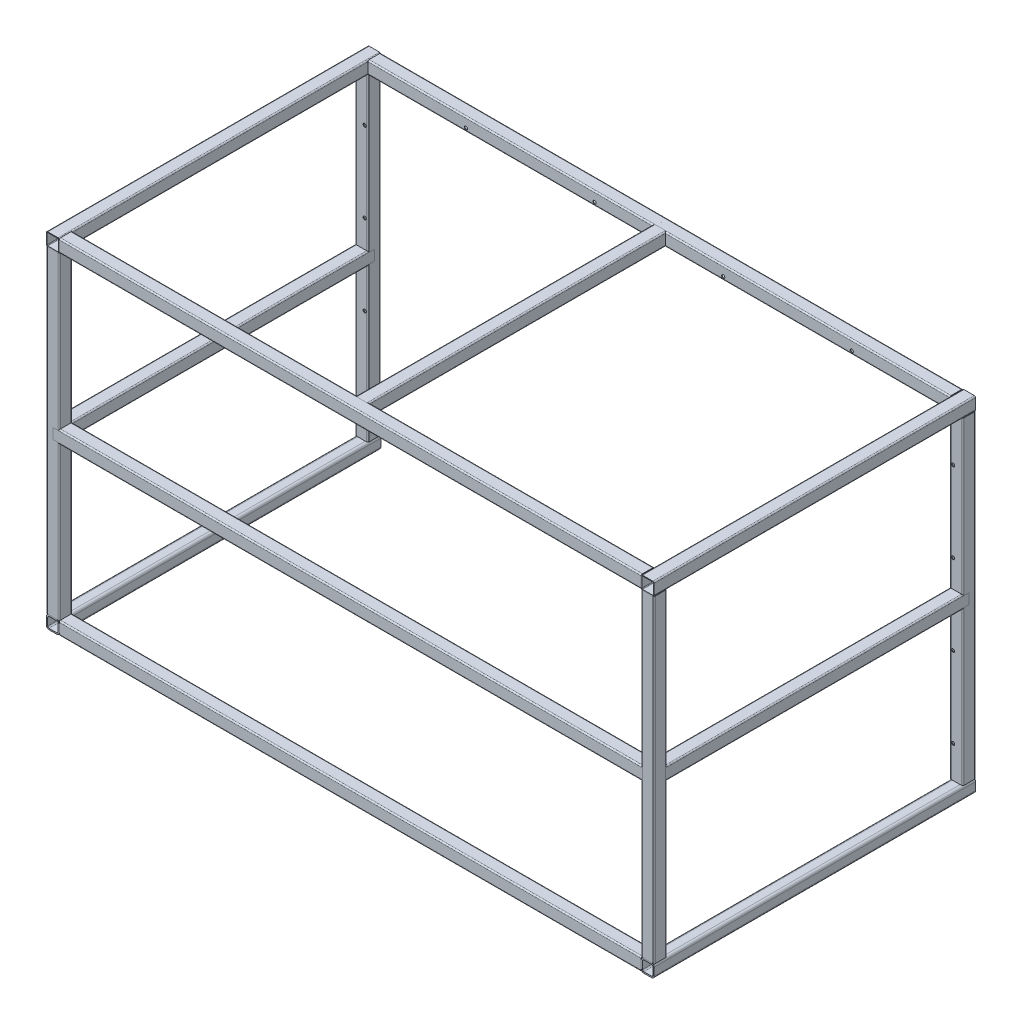
from build123d import *

# Parameters (mm, degrees)
SQUARE_TUBE_CONFIGURED_40_X_40_X_4_1_DEPTH      = 1870
SQUARE_TUBE_CONFIGURED_40_X_40_X_4_1_DEPTH_BACK = 1
SQUARE_TUBE_CONFIGURED_40_X_40_X_4_1_2_DEPTH    = 1051
SQUARE_TUBE_CONFIGURED_40_X_40_X_4_1_3_DEPTH    = 1871
SQUARE_TUBE_CONFIGURED_40_X_40_X_4_1_4_DEPTH    = 1051
SQUARE_TUBE_CONFIGURED_40_X_40_X_4_5_DEPTH      = 1050
SQUARE_TUBE_CONFIGURED_40_X_40_X_4_5_2_DEPTH    = 1871
SQUARE_TUBE_CONFIGURED_40_X_40_X_4_5_3_DEPTH    = 1031
SQUARE_TUBE_CONFIGURED_40_X_40_X_4_8_DEPTH      = 960
SQUARE_TUBE_CONFIGURED_40_X_40_X_4_8_2_DEPTH    = 960
BODY_START                                      = 134.13708499
BODY_4_RUN_ON_DEPTH                             = 153.13708499
BODY_7_RUN_ON_DEPTH                             = 153.13708499
BODY_2_RUN_ON_DEPTH                             = 153.13708499
BODY_START_2                                    = 113.13708499
BODY_8_RUN_ON_DEPTH                             = 133.13708499
BODY_START_3                                    = 846.86291501
BODY_8_RUN_ON_2_DEPTH                           = 133.13708499
BODY_9_RUN_ON_DEPTH                             = 133.13708499
BODY_9_RUN_ON_2_DEPTH                           = 133.13708499
SQUARE_TUBE_CONFIGURED_40_X_40_X_4_9_DEPTH      = 960
SQUARE_TUBE_CONFIGURED_40_X_40_X_4_10_DEPTH     = 1850
SQUARE_TUBE_CONFIGURED_40_X_40_X_4_11_DEPTH     = 960
SQUARE_TUBE_CONFIGURED_40_X_40_X_4_12_DEPTH     = 960
SQUARE_TUBE_CONFIGURED_40_X_40_X_4_13_DEPTH     = 670
SQUARE_TUBE_CONFIGURED_40_X_40_X_4_14_DEPTH     = 670
BODY_14_RUN_ON_DEPTH                            = 20
BODY_15_RUN_ON_DEPTH                            = 20
BODY_START_4                                    = 670
BODY_14_RUN_ON_2_DEPTH                          = 310
BODY_15_RUN_ON_2_DEPTH                          = 310
SKETCH_4_W                                      = 5
SKETCH_4_H                                      = 40
PATTERN_LINEAR_1_COUNT                          = 4
PATTERN_LINEAR_1_PITCH                          = 250
PATTERN_LINEAR_2_COUNT                          = 2
PATTERN_LINEAR_2_PITCH                          = 1830
PATTERN_LINEAR_2_COPY_1_SKETCH_W                = 5
PATTERN_LINEAR_2_COPY_1_SKETCH_H                = 40
PATTERN_LINEAR_2_COPY_2_SKETCH_W                = 5
PATTERN_LINEAR_2_COPY_2_SKETCH_H                = 40
PATTERN_LINEAR_2_COPY_3_SKETCH_W                = 5
PATTERN_LINEAR_2_COPY_3_SKETCH_H                = 40
SKETCH_6_W                                      = 5
SKETCH_6_H                                      = 40
PATTERN_LINEAR_3_COUNT                          = 4
PATTERN_LINEAR_3_PITCH                          = 400


with BuildPart() as part:
    # Sketch1 → Square tube - configured 40 X 40 X 4(1) (new, two sides: drawn at the far end of the back side and taken through both)
    with BuildSketch(Plane(origin=(-925, 515, 0), x_dir=(0, 1, 0), z_dir=(1, 0, 0)).offset(-SQUARE_TUBE_CONFIGURED_40_X_40_X_4_1_DEPTH_BACK)):
        with BuildLine():
            Line((-16, -20), (16, -20))
            ThreePointArc((16, -20), (18.828427125, -18.828427125), (20, -16))
            Line((20, -16), (20, 16))
            ThreePointArc((20, 16), (18.828427125, 18.828427125), (16, 20))
            Line((16, 20), (-16, 20))
            ThreePointArc((-16, 20), (-18.828427125, 18.828427125), (-20, 16))
            Line((-20, 16), (-20, -16))
            ThreePointArc((-20, -16), (-18.828427125, -18.828427125), (-16, -20))
        make_face()
        with BuildLine():
            Line((-16, -18), (16, -18))
            ThreePointArc((16, -18), (17.414213562, -17.414213562), (18, -16))
            Line((18, -16), (18, 16))
            ThreePointArc((18, 16), (17.414213562, 17.414213562), (16, 18))
            Line((16, 18), (-16, 18))
            ThreePointArc((-16, 18), (-17.414213562, 17.414213562), (-18, 16))
            Line((-18, 16), (-18, -16))
            ThreePointArc((-18, -16), (-17.414213562, -17.414213562), (-16, -18))
        make_face(mode=Mode.SUBTRACT)
    extrude(amount=SQUARE_TUBE_CONFIGURED_40_X_40_X_4_1_DEPTH + SQUARE_TUBE_CONFIGURED_40_X_40_X_4_1_DEPTH_BACK)

    # Square tube - configured 40 X 40 X 4(1) e
    split(bisect_by=Plane(origin=(-905, 515, 0), x_dir=(0, 1, 0), z_dir=(1, 0, 0)), keep=Keep.TOP)

    # Weld Trim 17 7
    split(bisect_by=Plane(origin=(943, -20, 0), x_dir=(0, -1, 0), z_dir=(-1, 0, 0)), keep=Keep.TOP)

    # Weld Trim 17 12
    split(bisect_by=Plane(origin=(907, -20, 0), x_dir=(0, -1, 0), z_dir=(-1, 0, 0)), keep=Keep.TOP)

    # Weld Trim 17 13
    split(bisect_by=Plane(origin=(905, -20, 0), x_dir=(0, -1, 0), z_dir=(-1, 0, 0)), keep=Keep.TOP)


with BuildPart() as body_2:
    # Sketch1 on segment 2 (carried to segment 2) → Square tube - configured 40 X 40 X 4_1 2 (new body)
    with BuildSketch(Plane(origin=(925, 516, 0), x_dir=(1, 0, 0), z_dir=(0, -1, 0))):
        with BuildLine():
            Line((-16, -20), (16, -20))
            ThreePointArc((16, -20), (18.828427125, -18.828427125), (20, -16))
            Line((20, -16), (20, 16))
            ThreePointArc((20, 16), (18.828427125, 18.828427125), (16, 20))
            Line((16, 20), (-16, 20))
            ThreePointArc((-16, 20), (-18.828427125, 18.828427125), (-20, 16))
            Line((-20, 16), (-20, -16))
            ThreePointArc((-20, -16), (-18.828427125, -18.828427125), (-16, -20))
        make_face()
        with BuildLine():
            Line((-16, -18), (16, -18))
            ThreePointArc((16, -18), (17.414213562, -17.414213562), (18, -16))
            Line((18, -16), (18, 16))
            ThreePointArc((18, 16), (17.414213562, 17.414213562), (16, 18))
            Line((16, 18), (-16, 18))
            ThreePointArc((-16, 18), (-17.414213562, 17.414213562), (-18, 16))
            Line((-18, 16), (-18, -16))
            ThreePointArc((-18, -16), (-17.414213562, -17.414213562), (-16, -18))
        make_face(mode=Mode.SUBTRACT)
    extrude(amount=SQUARE_TUBE_CONFIGURED_40_X_40_X_4_1_2_DEPTH)

    # Square tube - configured 40 X 40 X 4 2
    split(bisect_by=Plane(origin=(925, 495, 0), x_dir=(1, 0, 0), z_dir=(0, -1, 0)), keep=Keep.TOP)

    # body 2 cut square before the run-on
    split(bisect_by=Plane(origin=(925, 381.86291501, 0), x_dir=(1, 0, 0), z_dir=(0, -1, 0)), keep=Keep.TOP)

    # Sketch1 on segment 2 (carried to segment 2) → body 2 run on (add)
    with BuildSketch(Plane(origin=(925, 516, 0), x_dir=(1, 0, 0), z_dir=(0, -1, 0)).offset(BODY_START)):
        with BuildLine():
            Line((-16, -20), (16, -20))
            ThreePointArc((16, -20), (18.828427125, -18.828427125), (20, -16))
            Line((20, -16), (20, 16))
            ThreePointArc((20, 16), (18.828427125, 18.828427125), (16, 20))
            Line((16, 20), (-16, 20))
            ThreePointArc((-16, 20), (-18.828427125, 18.828427125), (-20, 16))
            Line((-20, 16), (-20, -16))
            ThreePointArc((-20, -16), (-18.828427125, -18.828427125), (-16, -20))
        make_face()
        with BuildLine():
            Line((-16, -18), (16, -18))
            ThreePointArc((16, -18), (17.414213562, -17.414213562), (18, -16))
            Line((18, -16), (18, 16))
            ThreePointArc((18, 16), (17.414213562, 17.414213562), (16, 18))
            Line((16, 18), (-16, 18))
            ThreePointArc((-16, 18), (-17.414213562, 17.414213562), (-18, 16))
            Line((-18, 16), (-18, -16))
            ThreePointArc((-18, -16), (-17.414213562, -17.414213562), (-16, -18))
        make_face(mode=Mode.SUBTRACT)
    extrude(amount=-BODY_2_RUN_ON_DEPTH)

    # Weld Trim 25 5
    split(bisect_by=Plane(origin=(925, 495, -490), x_dir=(1, 0, 0), z_dir=(0, -1, 0)), keep=Keep.TOP)

    # Weld Trim 32
    split(bisect_by=Plane(origin=(925, -495, -335), x_dir=(-1, 0, 0), z_dir=(0, 1, 0)), keep=Keep.TOP)


with BuildPart() as body_3:
    # Sketch1 on segment 3 (carried to segment 3) → Square tube - configured 40 X 40 X 4_1 3 (new body)
    with BuildSketch(Plane(origin=(926, -515, 0), x_dir=(0, -1, 0), z_dir=(-1, 0, 0))):
        with BuildLine():
            Line((-16, -20), (16, -20))
            ThreePointArc((16, -20), (18.828427125, -18.828427125), (20, -16))
            Line((20, -16), (20, 16))
            ThreePointArc((20, 16), (18.828427125, 18.828427125), (16, 20))
            Line((16, 20), (-16, 20))
            ThreePointArc((-16, 20), (-18.828427125, 18.828427125), (-20, 16))
            Line((-20, 16), (-20, -16))
            ThreePointArc((-20, -16), (-18.828427125, -18.828427125), (-16, -20))
        make_face()
        with BuildLine():
            Line((-16, -18), (16, -18))
            ThreePointArc((16, -18), (17.414213562, -17.414213562), (18, -16))
            Line((18, -16), (18, 16))
            ThreePointArc((18, 16), (17.414213562, 17.414213562), (16, 18))
            Line((16, 18), (-16, 18))
            ThreePointArc((-16, 18), (-17.414213562, 17.414213562), (-18, 16))
            Line((-18, 16), (-18, -16))
            ThreePointArc((-18, -16), (-17.414213562, -17.414213562), (-16, -18))
        make_face(mode=Mode.SUBTRACT)
    extrude(amount=SQUARE_TUBE_CONFIGURED_40_X_40_X_4_1_3_DEPTH)

    # Square tube - configured 40 X 40 X 4 3
    split(bisect_by=Plane(origin=(905, -515, 0), x_dir=(0, -1, 0), z_dir=(-1, 0, 0)), keep=Keep.TOP)

    # Weld Trim 1 7
    split(bisect_by=Plane(origin=(-943, 20, 0), x_dir=(0, 1, 0), z_dir=(1, 0, 0)), keep=Keep.TOP)

    # Weld Trim 1 12
    split(bisect_by=Plane(origin=(-907, 20, 0), x_dir=(0, 1, 0), z_dir=(1, 0, 0)), keep=Keep.TOP)

    # Weld Trim 1 13
    split(bisect_by=Plane(origin=(-905, 20, 0), x_dir=(0, 1, 0), z_dir=(1, 0, 0)), keep=Keep.TOP)


with BuildPart() as body_4:
    # Sketch1 on segment 4 (carried to segment 4) → Square tube - configured 40 X 40 X 4_1 4 (new body)
    with BuildSketch(Plane(origin=(-925, -516, 0), x_dir=(-1, 0, 0), z_dir=(0, 1, 0))):
        with BuildLine():
            Line((-16, -20), (16, -20))
            ThreePointArc((16, -20), (18.828427125, -18.828427125), (20, -16))
            Line((20, -16), (20, 16))
            ThreePointArc((20, 16), (18.828427125, 18.828427125), (16, 20))
            Line((16, 20), (-16, 20))
            ThreePointArc((-16, 20), (-18.828427125, 18.828427125), (-20, 16))
            Line((-20, 16), (-20, -16))
            ThreePointArc((-20, -16), (-18.828427125, -18.828427125), (-16, -20))
        make_face()
        with BuildLine():
            Line((-16, -18), (16, -18))
            ThreePointArc((16, -18), (17.414213562, -17.414213562), (18, -16))
            Line((18, -16), (18, 16))
            ThreePointArc((18, 16), (17.414213562, 17.414213562), (16, 18))
            Line((16, 18), (-16, 18))
            ThreePointArc((-16, 18), (-17.414213562, 17.414213562), (-18, 16))
            Line((-18, 16), (-18, -16))
            ThreePointArc((-18, -16), (-17.414213562, -17.414213562), (-16, -18))
        make_face(mode=Mode.SUBTRACT)
    extrude(amount=SQUARE_TUBE_CONFIGURED_40_X_40_X_4_1_4_DEPTH)

    # Square tube - configured 40 X 40 X 4 4
    split(bisect_by=Plane(origin=(-925, -495, 0), x_dir=(-1, 0, 0), z_dir=(0, 1, 0)), keep=Keep.TOP)

    # body 4 cut square before the run-on
    split(bisect_by=Plane(origin=(-925, -381.86291501, 0), x_dir=(-1, 0, 0), z_dir=(0, 1, 0)), keep=Keep.TOP)

    # Sketch1 on segment 4 (carried to segment 4) → body 4 run on (add)
    with BuildSketch(Plane(origin=(-925, -516, 0), x_dir=(-1, 0, 0), z_dir=(0, 1, 0)).offset(BODY_START)):
        with BuildLine():
            Line((-16, -20), (16, -20))
            ThreePointArc((16, -20), (18.828427125, -18.828427125), (20, -16))
            Line((20, -16), (20, 16))
            ThreePointArc((20, 16), (18.828427125, 18.828427125), (16, 20))
            Line((16, 20), (-16, 20))
            ThreePointArc((-16, 20), (-18.828427125, 18.828427125), (-20, 16))
            Line((-20, 16), (-20, -16))
            ThreePointArc((-20, -16), (-18.828427125, -18.828427125), (-16, -20))
        make_face()
        with BuildLine():
            Line((-16, -18), (16, -18))
            ThreePointArc((16, -18), (17.414213562, -17.414213562), (18, -16))
            Line((18, -16), (18, 16))
            ThreePointArc((18, 16), (17.414213562, 17.414213562), (16, 18))
            Line((16, 18), (-16, 18))
            ThreePointArc((-16, 18), (-17.414213562, 17.414213562), (-18, 16))
            Line((-18, 16), (-18, -16))
            ThreePointArc((-18, -16), (-17.414213562, -17.414213562), (-16, -18))
        make_face(mode=Mode.SUBTRACT)
    extrude(amount=-BODY_4_RUN_ON_DEPTH)

    # Weld Trim 18 5
    split(bisect_by=Plane(origin=(-925, 495, -480), x_dir=(1, 0, 0), z_dir=(0, -1, 0)), keep=Keep.TOP)

    # Weld Trim 31
    split(bisect_by=Plane(origin=(-925, -495, -335), x_dir=(-1, 0, 0), z_dir=(0, 1, 0)), keep=Keep.TOP)


with BuildPart() as body_5:
    # Sketch11 → Square tube - configured 40 X 40 X 4 5 (new body)
    with BuildSketch(Plane(origin=(925, -515, -960), x_dir=(-1, 0, 0), z_dir=(0, 1, 0))):
        with BuildLine():
            Line((-16, -20), (16, -20))
            ThreePointArc((16, -20), (18.828427125, -18.828427125), (20, -16))
            Line((20, -16), (20, 16))
            ThreePointArc((20, 16), (18.828427125, 18.828427125), (16, 20))
            Line((16, 20), (-16, 20))
            ThreePointArc((-16, 20), (-18.828427125, 18.828427125), (-20, 16))
            Line((-20, 16), (-20, -16))
            ThreePointArc((-20, -16), (-18.828427125, -18.828427125), (-16, -20))
        make_face()
        with BuildLine():
            Line((-16, -18), (16, -18))
            ThreePointArc((16, -18), (17.414213562, -17.414213562), (18, -16))
            Line((18, -16), (18, 16))
            ThreePointArc((18, 16), (17.414213562, 17.414213562), (16, 18))
            Line((16, 18), (-16, 18))
            ThreePointArc((-16, 18), (-17.414213562, 17.414213562), (-18, 16))
            Line((-18, 16), (-18, -16))
            ThreePointArc((-18, -16), (-17.414213562, -17.414213562), (-16, -18))
        make_face(mode=Mode.SUBTRACT)
    extrude(amount=SQUARE_TUBE_CONFIGURED_40_X_40_X_4_5_DEPTH)

    # Weld Trim 23 5
    split(bisect_by=Plane(origin=(925, 495, -480), x_dir=(1, 0, 0), z_dir=(0, -1, 0)), keep=Keep.TOP)

    # Weld Trim 34
    split(bisect_by=Plane(origin=(925, -495, -325), x_dir=(-1, 0, 0), z_dir=(0, 1, 0)), keep=Keep.TOP)

    # 草图4 → Ø10.0 (10) 直径孔1 (revolve, cut)
    with BuildSketch(Plane(origin=(915, -395, -940), x_dir=(0, -1, 0), z_dir=(1, 0, 0))):
        with Locations((2.5, 20)):
            Rectangle(SKETCH_4_W, SKETCH_4_H)
    hole_wizard_10_0_10_1 = revolve(axis=Axis((915, -395, -933.65), (0, 0, -1)), mode=Mode.SUBTRACT)

    # 阵列(线性)1: Ø10.0 (10) 直径孔1 ×4
    with Locations(*[(0, i * PATTERN_LINEAR_1_PITCH, 0) for i in range(1, PATTERN_LINEAR_1_COUNT)]):
        add(hole_wizard_10_0_10_1, mode=Mode.SUBTRACT)


with BuildPart() as body_6:
    # Sketch11 on segment 2 (carried to segment 2) → Square tube - configured 40 X 40 X 4 5 2 (new body)
    with BuildSketch(Plane(origin=(926, 515, -960), x_dir=(0, -1, 0), z_dir=(-1, 0, 0))):
        with BuildLine():
            Line((-16, -20), (16, -20))
            ThreePointArc((16, -20), (18.828427125, -18.828427125), (20, -16))
            Line((20, -16), (20, 16))
            ThreePointArc((20, 16), (18.828427125, 18.828427125), (16, 20))
            Line((16, 20), (-16, 20))
            ThreePointArc((-16, 20), (-18.828427125, 18.828427125), (-20, 16))
            Line((-20, 16), (-20, -16))
            ThreePointArc((-20, -16), (-18.828427125, -18.828427125), (-16, -20))
        make_face()
        with BuildLine():
            Line((-16, -18), (16, -18))
            ThreePointArc((16, -18), (17.414213562, -17.414213562), (18, -16))
            Line((18, -16), (18, 16))
            ThreePointArc((18, 16), (17.414213562, 17.414213562), (16, 18))
            Line((16, 18), (-16, 18))
            ThreePointArc((-16, 18), (-17.414213562, 17.414213562), (-18, 16))
            Line((-18, 16), (-18, -16))
            ThreePointArc((-18, -16), (-17.414213562, -17.414213562), (-16, -18))
        make_face(mode=Mode.SUBTRACT)
    extrude(amount=SQUARE_TUBE_CONFIGURED_40_X_40_X_4_5_2_DEPTH)

    # Square tube - configured 40 X 40 X 4 6
    split(bisect_by=Plane(origin=(905, 515, -960), x_dir=(0, -1, 0), z_dir=(-1, 0, 0)), keep=Keep.TOP)

    # Weld Trim 5 7
    split(bisect_by=Plane(origin=(-905, -10, -960), x_dir=(0, 1, 0), z_dir=(1, 0, 0)), keep=Keep.TOP)

    # 草图6 → Ø10.0 (10) 直径孔2 (revolve, cut)
    with BuildSketch(Plane(origin=(600, 505, -940), x_dir=(0, -1, 0), z_dir=(1, 0, 0))):
        with Locations((2.5, 20)):
            Rectangle(SKETCH_6_W, SKETCH_6_H)
    hole_wizard_10_0_10_2 = revolve(axis=Axis((600, 505, -933.65), (0, 0, -1)), mode=Mode.SUBTRACT)

    # 阵列(线性)3: Ø10.0 (10) 直径孔2 ×4
    with Locations(*[(-i * PATTERN_LINEAR_3_PITCH, 0, 0) for i in range(1, PATTERN_LINEAR_3_COUNT)]):
        add(hole_wizard_10_0_10_2, mode=Mode.SUBTRACT)


with BuildPart() as body_7:
    # Sketch11 on segment 3 (carried to segment 3) → Square tube - configured 40 X 40 X 4 5 3 (new body)
    with BuildSketch(Plane(origin=(-925, 516, -960), x_dir=(1, 0, 0), z_dir=(0, -1, 0))):
        with BuildLine():
            Line((-16, -20), (16, -20))
            ThreePointArc((16, -20), (18.828427125, -18.828427125), (20, -16))
            Line((20, -16), (20, 16))
            ThreePointArc((20, 16), (18.828427125, 18.828427125), (16, 20))
            Line((16, 20), (-16, 20))
            ThreePointArc((-16, 20), (-18.828427125, 18.828427125), (-20, 16))
            Line((-20, 16), (-20, -16))
            ThreePointArc((-20, -16), (-18.828427125, -18.828427125), (-16, -20))
        make_face()
        with BuildLine():
            Line((-16, -18), (16, -18))
            ThreePointArc((16, -18), (17.414213562, -17.414213562), (18, -16))
            Line((18, -16), (18, 16))
            ThreePointArc((18, 16), (17.414213562, 17.414213562), (16, 18))
            Line((16, 18), (-16, 18))
            ThreePointArc((-16, 18), (-17.414213562, 17.414213562), (-18, 16))
            Line((-18, 16), (-18, -16))
            ThreePointArc((-18, -16), (-17.414213562, -17.414213562), (-16, -18))
        make_face(mode=Mode.SUBTRACT)
    extrude(amount=SQUARE_TUBE_CONFIGURED_40_X_40_X_4_5_3_DEPTH)

    # Square tube - configured 40 X 40 X 4 7
    split(bisect_by=Plane(origin=(-925, 495, -960), x_dir=(1, 0, 0), z_dir=(0, -1, 0)), keep=Keep.TOP)

    # body 7 cut square before the run-on
    split(bisect_by=Plane(origin=(-925, 381.86291501, -960), x_dir=(1, 0, 0), z_dir=(0, -1, 0)), keep=Keep.TOP)

    # Sketch11 on segment 3 (carried to segment 3) → body 7 run on (add)
    with BuildSketch(Plane(origin=(-925, 516, -960), x_dir=(1, 0, 0), z_dir=(0, -1, 0)).offset(BODY_START)):
        with BuildLine():
            Line((-16, -20), (16, -20))
            ThreePointArc((16, -20), (18.828427125, -18.828427125), (20, -16))
            Line((20, -16), (20, 16))
            ThreePointArc((20, 16), (18.828427125, 18.828427125), (16, 20))
            Line((16, 20), (-16, 20))
            ThreePointArc((-16, 20), (-18.828427125, 18.828427125), (-20, 16))
            Line((-20, 16), (-20, -16))
            ThreePointArc((-20, -16), (-18.828427125, -18.828427125), (-16, -20))
        make_face()
        with BuildLine():
            Line((-16, -18), (16, -18))
            ThreePointArc((16, -18), (17.414213562, -17.414213562), (18, -16))
            Line((18, -16), (18, 16))
            ThreePointArc((18, 16), (17.414213562, 17.414213562), (16, 18))
            Line((16, 18), (-16, 18))
            ThreePointArc((-16, 18), (-17.414213562, 17.414213562), (-18, 16))
            Line((-18, 16), (-18, -16))
            ThreePointArc((-18, -16), (-17.414213562, -17.414213562), (-16, -18))
        make_face(mode=Mode.SUBTRACT)
    extrude(amount=-BODY_7_RUN_ON_DEPTH)

    # Weld Trim 22 3
    split(bisect_by=Plane(origin=(-925, 533, -470), x_dir=(1, 0, 0), z_dir=(0, -1, 0)), keep=Keep.TOP)

    # Weld Trim 22 8
    split(bisect_by=Plane(origin=(-925, 497, -470), x_dir=(1, 0, 0), z_dir=(0, -1, 0)), keep=Keep.TOP)

    # Weld Trim 22 13
    split(bisect_by=Plane(origin=(-925, 495, -470), x_dir=(1, 0, 0), z_dir=(0, -1, 0)), keep=Keep.TOP)

    # Weld Trim 33
    split(bisect_by=Plane(origin=(-925, -495, -325), x_dir=(-1, 0, 0), z_dir=(0, 1, 0)), keep=Keep.TOP)

    # 阵列(线性)2: Ø10.0 (10) 直径孔1 ×2
    with Locations(*[(-i * PATTERN_LINEAR_2_PITCH, 0, 0) for i in range(1, PATTERN_LINEAR_2_COUNT)]):
        add(hole_wizard_10_0_10_1, mode=Mode.SUBTRACT)

    # 阵列(线性)2 copy 1 sketch → 阵列(线性)2 copy 1 (revolve, cut)
    with BuildSketch(Plane(origin=(-915, -145, -940), x_dir=(0, -1, 0), z_dir=(1, 0, 0))):
        with Locations((2.5, 20)):
            Rectangle(PATTERN_LINEAR_2_COPY_1_SKETCH_W, PATTERN_LINEAR_2_COPY_1_SKETCH_H)
    revolve(axis=Axis((-915, -145, -933.65), (0, 0, -1)), mode=Mode.SUBTRACT)

    # 阵列(线性)2 copy 2 sketch → 阵列(线性)2 copy 2 (revolve, cut)
    with BuildSketch(Plane(origin=(-915, 105, -940), x_dir=(0, -1, 0), z_dir=(1, 0, 0))):
        with Locations((2.5, 20)):
            Rectangle(PATTERN_LINEAR_2_COPY_2_SKETCH_W, PATTERN_LINEAR_2_COPY_2_SKETCH_H)
    revolve(axis=Axis((-915, 105, -933.65), (0, 0, -1)), mode=Mode.SUBTRACT)

    # 阵列(线性)2 copy 3 sketch → 阵列(线性)2 copy 3 (revolve, cut)
    with BuildSketch(Plane(origin=(-915, 355, -940), x_dir=(0, -1, 0), z_dir=(1, 0, 0))):
        with Locations((2.5, 20)):
            Rectangle(PATTERN_LINEAR_2_COPY_3_SKETCH_W, PATTERN_LINEAR_2_COPY_3_SKETCH_H)
    revolve(axis=Axis((-915, 355, -933.65), (0, 0, -1)), mode=Mode.SUBTRACT)


with BuildPart() as body_8:
    # Sketch12 → Square tube - configured 40 X 40 X 4 8 (new body)
    with BuildSketch(Plane(origin=(-925, 515, 0), x_dir=(1, 0, 0), z_dir=(0, 0, -1))):
        with BuildLine():
            Line((-16, -20), (16, -20))
            ThreePointArc((16, -20), (18.828427125, -18.828427125), (20, -16))
            Line((20, -16), (20, 16))
            ThreePointArc((20, 16), (18.828427125, 18.828427125), (16, 20))
            Line((16, 20), (-16, 20))
            ThreePointArc((-16, 20), (-18.828427125, 18.828427125), (-20, 16))
            Line((-20, 16), (-20, -16))
            ThreePointArc((-20, -16), (-18.828427125, -18.828427125), (-16, -20))
        make_face()
        with BuildLine():
            Line((-16, -18), (16, -18))
            ThreePointArc((16, -18), (17.414213562, -17.414213562), (18, -16))
            Line((18, -16), (18, 16))
            ThreePointArc((18, 16), (17.414213562, 17.414213562), (16, 18))
            Line((16, 18), (-16, 18))
            ThreePointArc((-16, 18), (-17.414213562, 17.414213562), (-18, 16))
            Line((-18, 16), (-18, -16))
            ThreePointArc((-18, -16), (-17.414213562, -17.414213562), (-16, -18))
        make_face(mode=Mode.SUBTRACT)
    extrude(amount=SQUARE_TUBE_CONFIGURED_40_X_40_X_4_8_DEPTH)

    # body 8 cut square before the run-on
    split(bisect_by=Plane(origin=(-925, 515, -113.13708499), x_dir=(0, 1, 0), z_dir=(0, 0, -1)), keep=Keep.TOP)

    # Sketch12 → body 8 run on (add)
    with BuildSketch(Plane(origin=(-925, 515, 0), x_dir=(1, 0, 0), z_dir=(0, 0, -1)).offset(BODY_START_2)):
        with BuildLine():
            Line((-16, -20), (16, -20))
            ThreePointArc((16, -20), (18.828427125, -18.828427125), (20, -16))
            Line((20, -16), (20, 16))
            ThreePointArc((20, 16), (18.828427125, 18.828427125), (16, 20))
            Line((16, 20), (-16, 20))
            ThreePointArc((-16, 20), (-18.828427125, 18.828427125), (-20, 16))
            Line((-20, 16), (-20, -16))
            ThreePointArc((-20, -16), (-18.828427125, -18.828427125), (-16, -20))
        make_face()
        with BuildLine():
            Line((-16, -18), (16, -18))
            ThreePointArc((16, -18), (17.414213562, -17.414213562), (18, -16))
            Line((18, -16), (18, 16))
            ThreePointArc((18, 16), (17.414213562, 17.414213562), (16, 18))
            Line((16, 18), (-16, 18))
            ThreePointArc((-16, 18), (-17.414213562, 17.414213562), (-18, 16))
            Line((-18, 16), (-18, -16))
            ThreePointArc((-18, -16), (-17.414213562, -17.414213562), (-16, -18))
        make_face(mode=Mode.SUBTRACT)
    extrude(amount=-BODY_8_RUN_ON_DEPTH)

    # body 8 cut square before the run-on
    split(bisect_by=Plane(origin=(-925, 515, -846.86291501), x_dir=(0, -1, 0), z_dir=(0, 0, 1)), keep=Keep.TOP)

    # Sketch12 → body 8 run on 2 (add)
    with BuildSketch(Plane(origin=(-925, 515, 0), x_dir=(1, 0, 0), z_dir=(0, 0, -1)).offset(BODY_START_3)):
        with BuildLine():
            Line((-16, -20), (16, -20))
            ThreePointArc((16, -20), (18.828427125, -18.828427125), (20, -16))
            Line((20, -16), (20, 16))
            ThreePointArc((20, 16), (18.828427125, 18.828427125), (16, 20))
            Line((16, 20), (-16, 20))
            ThreePointArc((-16, 20), (-18.828427125, 18.828427125), (-20, 16))
            Line((-20, 16), (-20, -16))
            ThreePointArc((-20, -16), (-18.828427125, -18.828427125), (-16, -20))
        make_face()
        with BuildLine():
            Line((-16, -18), (16, -18))
            ThreePointArc((16, -18), (17.414213562, -17.414213562), (18, -16))
            Line((18, -16), (18, 16))
            ThreePointArc((18, 16), (17.414213562, 17.414213562), (16, 18))
            Line((16, 18), (-16, 18))
            ThreePointArc((-16, 18), (-17.414213562, 17.414213562), (-18, 16))
            Line((-18, 16), (-18, -16))
            ThreePointArc((-18, -16), (-17.414213562, -17.414213562), (-16, -18))
        make_face(mode=Mode.SUBTRACT)
    extrude(amount=BODY_8_RUN_ON_2_DEPTH)


with BuildPart() as body_9:
    # Sketch12 on segment 2 (carried to segment 2) → Square tube - configured 40 X 40 X 4 8 2 (new body)
    with BuildSketch(Plane(origin=(925, 515, 0), x_dir=(1, 0, 0), z_dir=(0, 0, -1))):
        with BuildLine():
            Line((-16, -20), (16, -20))
            ThreePointArc((16, -20), (18.828427125, -18.828427125), (20, -16))
            Line((20, -16), (20, 16))
            ThreePointArc((20, 16), (18.828427125, 18.828427125), (16, 20))
            Line((16, 20), (-16, 20))
            ThreePointArc((-16, 20), (-18.828427125, 18.828427125), (-20, 16))
            Line((-20, 16), (-20, -16))
            ThreePointArc((-20, -16), (-18.828427125, -18.828427125), (-16, -20))
        make_face()
        with BuildLine():
            Line((-16, -18), (16, -18))
            ThreePointArc((16, -18), (17.414213562, -17.414213562), (18, -16))
            Line((18, -16), (18, 16))
            ThreePointArc((18, 16), (17.414213562, 17.414213562), (16, 18))
            Line((16, 18), (-16, 18))
            ThreePointArc((-16, 18), (-17.414213562, 17.414213562), (-18, 16))
            Line((-18, 16), (-18, -16))
            ThreePointArc((-18, -16), (-17.414213562, -17.414213562), (-16, -18))
        make_face(mode=Mode.SUBTRACT)
    extrude(amount=SQUARE_TUBE_CONFIGURED_40_X_40_X_4_8_2_DEPTH)

    # body 9 cut square before the run-on
    split(bisect_by=Plane(origin=(925, 515, -846.86291501), x_dir=(0, -1, 0), z_dir=(0, 0, 1)), keep=Keep.TOP)

    # Sketch12 on segment 2 (carried to segment 2) → body 9 run on (add)
    with BuildSketch(Plane(origin=(925, 515, 0), x_dir=(1, 0, 0), z_dir=(0, 0, -1)).offset(BODY_START_3)):
        with BuildLine():
            Line((-16, -20), (16, -20))
            ThreePointArc((16, -20), (18.828427125, -18.828427125), (20, -16))
            Line((20, -16), (20, 16))
            ThreePointArc((20, 16), (18.828427125, 18.828427125), (16, 20))
            Line((16, 20), (-16, 20))
            ThreePointArc((-16, 20), (-18.828427125, 18.828427125), (-20, 16))
            Line((-20, 16), (-20, -16))
            ThreePointArc((-20, -16), (-18.828427125, -18.828427125), (-16, -20))
        make_face()
        with BuildLine():
            Line((-16, -18), (16, -18))
            ThreePointArc((16, -18), (17.414213562, -17.414213562), (18, -16))
            Line((18, -16), (18, 16))
            ThreePointArc((18, 16), (17.414213562, 17.414213562), (16, 18))
            Line((16, 18), (-16, 18))
            ThreePointArc((-16, 18), (-17.414213562, 17.414213562), (-18, 16))
            Line((-18, 16), (-18, -16))
            ThreePointArc((-18, -16), (-17.414213562, -17.414213562), (-16, -18))
        make_face(mode=Mode.SUBTRACT)
    extrude(amount=BODY_9_RUN_ON_DEPTH)

    # body 9 cut square before the run-on
    split(bisect_by=Plane(origin=(925, 515, -113.13708499), x_dir=(0, 1, 0), z_dir=(0, 0, -1)), keep=Keep.TOP)

    # Sketch12 on segment 2 (carried to segment 2) → body 9 run on 2 (add)
    with BuildSketch(Plane(origin=(925, 515, 0), x_dir=(1, 0, 0), z_dir=(0, 0, -1)).offset(BODY_START_2)):
        with BuildLine():
            Line((-16, -20), (16, -20))
            ThreePointArc((16, -20), (18.828427125, -18.828427125), (20, -16))
            Line((20, -16), (20, 16))
            ThreePointArc((20, 16), (18.828427125, 18.828427125), (16, 20))
            Line((16, 20), (-16, 20))
            ThreePointArc((-16, 20), (-18.828427125, 18.828427125), (-20, 16))
            Line((-20, 16), (-20, -16))
            ThreePointArc((-20, -16), (-18.828427125, -18.828427125), (-16, -20))
        make_face()
        with BuildLine():
            Line((-16, -18), (16, -18))
            ThreePointArc((16, -18), (17.414213562, -17.414213562), (18, -16))
            Line((18, -16), (18, 16))
            ThreePointArc((18, 16), (17.414213562, 17.414213562), (16, 18))
            Line((16, 18), (-16, 18))
            ThreePointArc((-16, 18), (-17.414213562, 17.414213562), (-18, 16))
            Line((-18, 16), (-18, -16))
            ThreePointArc((-18, -16), (-17.414213562, -17.414213562), (-16, -18))
        make_face(mode=Mode.SUBTRACT)
    extrude(amount=-BODY_9_RUN_ON_2_DEPTH)


with BuildPart() as body_10:
    # Sketch14 → Square tube - configured 40 X 40 X 4 9 (new body)
    with BuildSketch(Plane(origin=(0, 515, -960), x_dir=(1, 0, 0), z_dir=(0, 0, 1))):
        with BuildLine():
            Line((-16, -20), (16, -20))
            ThreePointArc((16, -20), (18.828427125, -18.828427125), (20, -16))
            Line((20, -16), (20, 16))
            ThreePointArc((20, 16), (18.828427125, 18.828427125), (16, 20))
            Line((16, 20), (-16, 20))
            ThreePointArc((-16, 20), (-18.828427125, 18.828427125), (-20, 16))
            Line((-20, 16), (-20, -16))
            ThreePointArc((-20, -16), (-18.828427125, -18.828427125), (-16, -20))
        make_face()
        with BuildLine():
            Line((-16, -18), (16, -18))
            ThreePointArc((16, -18), (17.414213562, -17.414213562), (18, -16))
            Line((18, -16), (18, 16))
            ThreePointArc((18, 16), (17.414213562, 17.414213562), (16, 18))
            Line((16, 18), (-16, 18))
            ThreePointArc((-16, 18), (-17.414213562, 17.414213562), (-18, 16))
            Line((-18, 16), (-18, -16))
            ThreePointArc((-18, -16), (-17.414213562, -17.414213562), (-16, -18))
        make_face(mode=Mode.SUBTRACT)
    extrude(amount=SQUARE_TUBE_CONFIGURED_40_X_40_X_4_9_DEPTH)


with BuildPart() as body_11:
    # Sketch15 → Square tube - configured 40 X 40 X 4 10 (new body)
    with BuildSketch(Plane.ZY.offset(-925)):
        with BuildLine():
            Line((-16, -20), (16, -20))
            ThreePointArc((16, -20), (18.828427125, -18.828427125), (20, -16))
            Line((20, -16), (20, 16))
            ThreePointArc((20, 16), (18.828427125, 18.828427125), (16, 20))
            Line((16, 20), (-16, 20))
            ThreePointArc((-16, 20), (-18.828427125, 18.828427125), (-20, 16))
            Line((-20, 16), (-20, -16))
            ThreePointArc((-20, -16), (-18.828427125, -18.828427125), (-16, -20))
        make_face()
        with BuildLine():
            Line((-16, -18), (16, -18))
            ThreePointArc((16, -18), (17.414213562, -17.414213562), (18, -16))
            Line((18, -16), (18, 16))
            ThreePointArc((18, 16), (17.414213562, 17.414213562), (16, 18))
            Line((16, 18), (-16, 18))
            ThreePointArc((-16, 18), (-17.414213562, 17.414213562), (-18, 16))
            Line((-18, 16), (-18, -16))
            ThreePointArc((-18, -16), (-17.414213562, -17.414213562), (-16, -18))
        make_face(mode=Mode.SUBTRACT)
    extrude(amount=SQUARE_TUBE_CONFIGURED_40_X_40_X_4_10_DEPTH)


with BuildPart() as body_12:
    # Sketch16 → Square tube - configured 40 X 40 X 4 11 (new body)
    with BuildSketch(Plane(origin=(-925, 0, 0), x_dir=(1, 0, 0), z_dir=(0, 0, -1))):
        with BuildLine():
            Line((-16, -20), (16, -20))
            ThreePointArc((16, -20), (18.828427125, -18.828427125), (20, -16))
            Line((20, -16), (20, 16))
            ThreePointArc((20, 16), (18.828427125, 18.828427125), (16, 20))
            Line((16, 20), (-16, 20))
            ThreePointArc((-16, 20), (-18.828427125, 18.828427125), (-20, 16))
            Line((-20, 16), (-20, -16))
            ThreePointArc((-20, -16), (-18.828427125, -18.828427125), (-16, -20))
        make_face()
        with BuildLine():
            Line((-16, -18), (16, -18))
            ThreePointArc((16, -18), (17.414213562, -17.414213562), (18, -16))
            Line((18, -16), (18, 16))
            ThreePointArc((18, 16), (17.414213562, 17.414213562), (16, 18))
            Line((16, 18), (-16, 18))
            ThreePointArc((-16, 18), (-17.414213562, 17.414213562), (-18, 16))
            Line((-18, 16), (-18, -16))
            ThreePointArc((-18, -16), (-17.414213562, -17.414213562), (-16, -18))
        make_face(mode=Mode.SUBTRACT)
    extrude(amount=SQUARE_TUBE_CONFIGURED_40_X_40_X_4_11_DEPTH)


with BuildPart() as body_13:
    # Sketch16 on segment 2 (carried to segment 2) → Square tube - configured 40 X 40 X 4 12 (new body)
    with BuildSketch(Plane(origin=(925, 0, 0), x_dir=(1, 0, 0), z_dir=(0, 0, -1))):
        with BuildLine():
            Line((-16, -20), (16, -20))
            ThreePointArc((16, -20), (18.828427125, -18.828427125), (20, -16))
            Line((20, -16), (20, 16))
            ThreePointArc((20, 16), (18.828427125, 18.828427125), (16, 20))
            Line((16, 20), (-16, 20))
            ThreePointArc((-16, 20), (-18.828427125, 18.828427125), (-20, 16))
            Line((-20, 16), (-20, -16))
            ThreePointArc((-20, -16), (-18.828427125, -18.828427125), (-16, -20))
        make_face()
        with BuildLine():
            Line((-16, -18), (16, -18))
            ThreePointArc((16, -18), (17.414213562, -17.414213562), (18, -16))
            Line((18, -16), (18, 16))
            ThreePointArc((18, 16), (17.414213562, 17.414213562), (16, 18))
            Line((16, 18), (-16, 18))
            ThreePointArc((-16, 18), (-17.414213562, 17.414213562), (-18, 16))
            Line((-18, 16), (-18, -16))
            ThreePointArc((-18, -16), (-17.414213562, -17.414213562), (-16, -18))
        make_face(mode=Mode.SUBTRACT)
    extrude(amount=SQUARE_TUBE_CONFIGURED_40_X_40_X_4_12_DEPTH)


with BuildPart() as body_14:
    # Sketch17 → Square tube - configured 40 X 40 X 4 13 (new body)
    with BuildSketch(Plane(origin=(-925, -515, 0), x_dir=(1, 0, 0), z_dir=(0, 0, -1))):
        with BuildLine():
            Line((-12, -20), (12, -20))
            ThreePointArc((12, -20), (17.656854249, -17.656854249), (20, -12))
            Line((20, -12), (20, 12))
            ThreePointArc((20, 12), (17.656854249, 17.656854249), (12, 20))
            Line((12, 20), (-12, 20))
            ThreePointArc((-12, 20), (-17.656854249, 17.656854249), (-20, 12))
            Line((-20, 12), (-20, -12))
            ThreePointArc((-20, -12), (-17.656854249, -17.656854249), (-12, -20))
        make_face()
        with BuildLine():
            Line((-12, -16), (12, -16))
            ThreePointArc((12, -16), (14.828427125, -14.828427125), (16, -12))
            Line((16, -12), (16, 12))
            ThreePointArc((16, 12), (14.828427125, 14.828427125), (12, 16))
            Line((12, 16), (-12, 16))
            ThreePointArc((-12, 16), (-14.828427125, 14.828427125), (-16, 12))
            Line((-16, 12), (-16, -12))
            ThreePointArc((-16, -12), (-14.828427125, -14.828427125), (-12, -16))
        make_face(mode=Mode.SUBTRACT)
    extrude(amount=SQUARE_TUBE_CONFIGURED_40_X_40_X_4_13_DEPTH)

    # Sketch17 → body 14 run on (add)
    with BuildSketch(Plane(origin=(-925, -515, 0), x_dir=(1, 0, 0), z_dir=(0, 0, -1))):
        with BuildLine():
            Line((-12, -20), (12, -20))
            ThreePointArc((12, -20), (17.656854249, -17.656854249), (20, -12))
            Line((20, -12), (20, 12))
            ThreePointArc((20, 12), (17.656854249, 17.656854249), (12, 20))
            Line((12, 20), (-12, 20))
            ThreePointArc((-12, 20), (-17.656854249, 17.656854249), (-20, 12))
            Line((-20, 12), (-20, -12))
            ThreePointArc((-20, -12), (-17.656854249, -17.656854249), (-12, -20))
        make_face()
        with BuildLine():
            Line((-12, -16), (12, -16))
            ThreePointArc((12, -16), (14.828427125, -14.828427125), (16, -12))
            Line((16, -12), (16, 12))
            ThreePointArc((16, 12), (14.828427125, 14.828427125), (12, 16))
            Line((12, 16), (-12, 16))
            ThreePointArc((-12, 16), (-14.828427125, 14.828427125), (-16, 12))
            Line((-16, 12), (-16, -12))
            ThreePointArc((-16, -12), (-14.828427125, -14.828427125), (-12, -16))
        make_face(mode=Mode.SUBTRACT)
    extrude(amount=-BODY_14_RUN_ON_DEPTH)

    # Sketch17 → body 14 run on 2 (add)
    with BuildSketch(Plane(origin=(-925, -515, 0), x_dir=(1, 0, 0), z_dir=(0, 0, -1)).offset(BODY_START_4)):
        with BuildLine():
            Line((-12, -20), (12, -20))
            ThreePointArc((12, -20), (17.656854249, -17.656854249), (20, -12))
            Line((20, -12), (20, 12))
            ThreePointArc((20, 12), (17.656854249, 17.656854249), (12, 20))
            Line((12, 20), (-12, 20))
            ThreePointArc((-12, 20), (-17.656854249, 17.656854249), (-20, 12))
            Line((-20, 12), (-20, -12))
            ThreePointArc((-20, -12), (-17.656854249, -17.656854249), (-12, -20))
        make_face()
        with BuildLine():
            Line((-12, -16), (12, -16))
            ThreePointArc((12, -16), (14.828427125, -14.828427125), (16, -12))
            Line((16, -12), (16, 12))
            ThreePointArc((16, 12), (14.828427125, 14.828427125), (12, 16))
            Line((12, 16), (-12, 16))
            ThreePointArc((-12, 16), (-14.828427125, 14.828427125), (-16, 12))
            Line((-16, 12), (-16, -12))
            ThreePointArc((-16, -12), (-14.828427125, -14.828427125), (-12, -16))
        make_face(mode=Mode.SUBTRACT)
    extrude(amount=BODY_14_RUN_ON_2_DEPTH)


with BuildPart() as body_15:
    # Sketch17 on segment 2 (carried to segment 2) → Square tube - configured 40 X 40 X 4 14 (new body)
    with BuildSketch(Plane(origin=(925, -515, 0), x_dir=(1, 0, 0), z_dir=(0, 0, -1))):
        with BuildLine():
            Line((-12, -20), (12, -20))
            ThreePointArc((12, -20), (17.656854249, -17.656854249), (20, -12))
            Line((20, -12), (20, 12))
            ThreePointArc((20, 12), (17.656854249, 17.656854249), (12, 20))
            Line((12, 20), (-12, 20))
            ThreePointArc((-12, 20), (-17.656854249, 17.656854249), (-20, 12))
            Line((-20, 12), (-20, -12))
            ThreePointArc((-20, -12), (-17.656854249, -17.656854249), (-12, -20))
        make_face()
        with BuildLine():
            Line((-12, -16), (12, -16))
            ThreePointArc((12, -16), (14.828427125, -14.828427125), (16, -12))
            Line((16, -12), (16, 12))
            ThreePointArc((16, 12), (14.828427125, 14.828427125), (12, 16))
            Line((12, 16), (-12, 16))
            ThreePointArc((-12, 16), (-14.828427125, 14.828427125), (-16, 12))
            Line((-16, 12), (-16, -12))
            ThreePointArc((-16, -12), (-14.828427125, -14.828427125), (-12, -16))
        make_face(mode=Mode.SUBTRACT)
    extrude(amount=SQUARE_TUBE_CONFIGURED_40_X_40_X_4_14_DEPTH)

    # Sketch17 on segment 2 (carried to segment 2) → body 15 run on (add)
    with BuildSketch(Plane(origin=(925, -515, 0), x_dir=(1, 0, 0), z_dir=(0, 0, -1))):
        with BuildLine():
            Line((-12, -20), (12, -20))
            ThreePointArc((12, -20), (17.656854249, -17.656854249), (20, -12))
            Line((20, -12), (20, 12))
            ThreePointArc((20, 12), (17.656854249, 17.656854249), (12, 20))
            Line((12, 20), (-12, 20))
            ThreePointArc((-12, 20), (-17.656854249, 17.656854249), (-20, 12))
            Line((-20, 12), (-20, -12))
            ThreePointArc((-20, -12), (-17.656854249, -17.656854249), (-12, -20))
        make_face()
        with BuildLine():
            Line((-12, -16), (12, -16))
            ThreePointArc((12, -16), (14.828427125, -14.828427125), (16, -12))
            Line((16, -12), (16, 12))
            ThreePointArc((16, 12), (14.828427125, 14.828427125), (12, 16))
            Line((12, 16), (-12, 16))
            ThreePointArc((-12, 16), (-14.828427125, 14.828427125), (-16, 12))
            Line((-16, 12), (-16, -12))
            ThreePointArc((-16, -12), (-14.828427125, -14.828427125), (-12, -16))
        make_face(mode=Mode.SUBTRACT)
    extrude(amount=-BODY_15_RUN_ON_DEPTH)

    # Sketch17 on segment 2 (carried to segment 2) → body 15 run on 2 (add)
    with BuildSketch(Plane(origin=(925, -515, 0), x_dir=(1, 0, 0), z_dir=(0, 0, -1)).offset(BODY_START_4)):
        with BuildLine():
            Line((-12, -20), (12, -20))
            ThreePointArc((12, -20), (17.656854249, -17.656854249), (20, -12))
            Line((20, -12), (20, 12))
            ThreePointArc((20, 12), (17.656854249, 17.656854249), (12, 20))
            Line((12, 20), (-12, 20))
            ThreePointArc((-12, 20), (-17.656854249, 17.656854249), (-20, 12))
            Line((-20, 12), (-20, -12))
            ThreePointArc((-20, -12), (-17.656854249, -17.656854249), (-12, -20))
        make_face()
        with BuildLine():
            Line((-12, -16), (12, -16))
            ThreePointArc((12, -16), (14.828427125, -14.828427125), (16, -12))
            Line((16, -12), (16, 12))
            ThreePointArc((16, 12), (14.828427125, 14.828427125), (12, 16))
            Line((12, 16), (-12, 16))
            ThreePointArc((-12, 16), (-14.828427125, 14.828427125), (-16, 12))
            Line((-16, 12), (-16, -12))
            ThreePointArc((-16, -12), (-14.828427125, -14.828427125), (-12, -16))
        make_face(mode=Mode.SUBTRACT)
    extrude(amount=BODY_15_RUN_ON_2_DEPTH)


solid = Compound([part.part, body_2.part, body_3.part, body_4.part, body_5.part, body_6.part, body_7.part, body_8.part, body_9.part, body_10.part, body_11.part, body_12.part, body_13.part, body_14.part, body_15.part])
